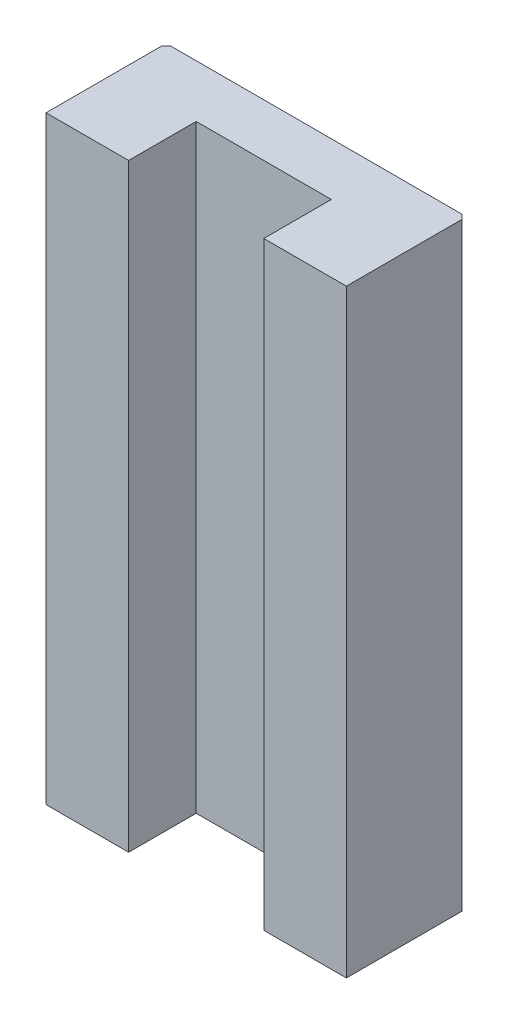
SolidWorks part; units mm, degrees
ref_plane "Front Plane" through (0, 0, 0) normal (0, 0, 1) x (1, 0, 0)
ref_plane "Top Plane" through (0, 0, 0) normal (0, 1, 0) x (1, 0, 0)
ref_plane "Right Plane" through (0, 0, 0) normal (1, 0, 0) x (0, 0, -1)
sketch "Sketch1" plane through (0, 0, 0) normal (0, 1, 0) x (1, 0, 0)
  line L0 (0, 0) -> (0, -50000) construction
  line L1 (-10, 4) -> (10, 4)
  line L2 (-10, 4) -> (-10, -4)
  line L3 (-10, -4) -> (10, -4)
  line L4 (10, 4) -> (10, -4)
  line L5 (-10, 4) -> (10, -4) construction
  line L6 (-10, -4) -> (10, 4) construction
  point P0 (0, 0)
  dimension "D1" = 20
  dimension "D2" = 8
extrude "Boss-Extrude1" add sketch "Sketch1" along normal blind 39.9
sketch "Sketch2" plane through (0, 39.9, 0) normal (0, 1, 0) x (1, 0, 0)
  line L0 (0, 0) -> (0, -50000) construction
  line L1 (-10, -4) -> (10, -4) construction
  line L2 (-4.5, -8.5) -> (4.5, -8.5)
  line L3 (-4.5, -8.5) -> (-4.5, 0.5)
  line L4 (-4.5, 0.5) -> (4.5, 0.5)
  line L5 (4.5, -8.5) -> (4.5, 0.5)
  line L6 (-4.5, -8.5) -> (4.5, 0.5) construction
  line L7 (-4.5, 0.5) -> (4.5, -8.5) construction
  point P3 (0, -4)
  dimension "D1" = 9
  dimension "D2" = 4.5
extrude "Cut-Extrude1" cut sketch "Sketch2" against normal through all
chamfer "Chamfer1" distance 0.3 angle 45 2 edges at (-10, 19.95, -4) (10, 19.95, -4)
sketch "Sketch3" plane through (0, 0, -4) normal (0, 0, -1) x (-1, 0, 0)
  line L0 (0, 0) -> (0, 50000) construction
  line L1 (-10, 19.95) -> (49990, 19.95) construction
  line L2 (-10, 0) -> (-10, 39.9) construction
  line L3 (10, 39.9) -> (10, 0) construction
  circle A0 centre (-7.5, 27.95) radius 0.593
  circle A1 centre (7.5, 27.95) radius 0.593
  circle A2 centre (7.5, 11.95) radius 0.593
  circle A3 centre (-7.5, 11.95) radius 0.593
  point P7 (-10, 19.95)
  point P10 (10, 19.95)
  dimension "D2" = 16
  dimension "D1" = 15
extrude "Cut-Extrude2" cut sketch "Sketch3" against normal blind 3
sketch "Sketch4" plane through (0, 0, 0) normal (0, -1, 0) x (1, 0, 0)
  line L0 (0, 0) -> (0, -50000) construction
  line L1 (9.7, -4) -> (-9.7, -4) construction
  circle A0 centre (0, -2.2) radius 0.6
  dimension "D1" = 1.2
  dimension "D2" = 1.8
extrude "Cut-Extrude3" cut sketch "Sketch4" against normal blind 4.5
hole_wizard "M3 Tapped Hole1" positions "3DSketch1" profile "Sketch5" tap size "M3" standard "Gb"
sketch3d "3DSketch1"
  line L0 (7.5, 11.95, -1) -> (7.5, 11.95, -4) construction
  line L1 (-7.5, 11.95, -1) -> (-7.5, 11.95, -4) construction
  line L2 (-7.5, 27.95, -1) -> (-7.5, 27.95, -4) construction
  line L3 (7.5, 27.95, -1) -> (7.5, 27.95, -4) construction
  point P0 (7.5, 11.95, -4)
  point P4 (-7.5, 11.95, -4)
  point P8 (-7.5, 27.95, -4)
  point P12 (7.5, 27.95, -4)
sketch "Sketch5" plane through (7.5, 11.95, -4) normal (1, 0, 0) x (0, 1, 0)
  line L0 (0, 0) -> (0, 5.7511)
  line L1 (0, 5.7511) -> (1.25, 5)
  line L2 (1.25, 5) -> (1.25, 0)
  line L5 (1.25, 0) -> (0, 0)
  line L10 (0, 5.7511) -> (-1.25, 5) construction
  line L11 (0, -6.35) -> (0, 107.95) construction
  dimension "螺纹孔钻头直径" = 2.5
  dimension "螺纹孔钻头深度" = 5
  dimension "导头角度" = 118
cosmetic thread "Cosmetic Thread1" parameters "D1"=5, "D2"=3
cosmetic thread "Cosmetic Thread2" parameters "D1"=5, "D2"=3
cosmetic thread "Cosmetic Thread3" parameters "D1"=5, "D2"=3
cosmetic thread "Cosmetic Thread4" parameters "D1"=5, "D2"=3
